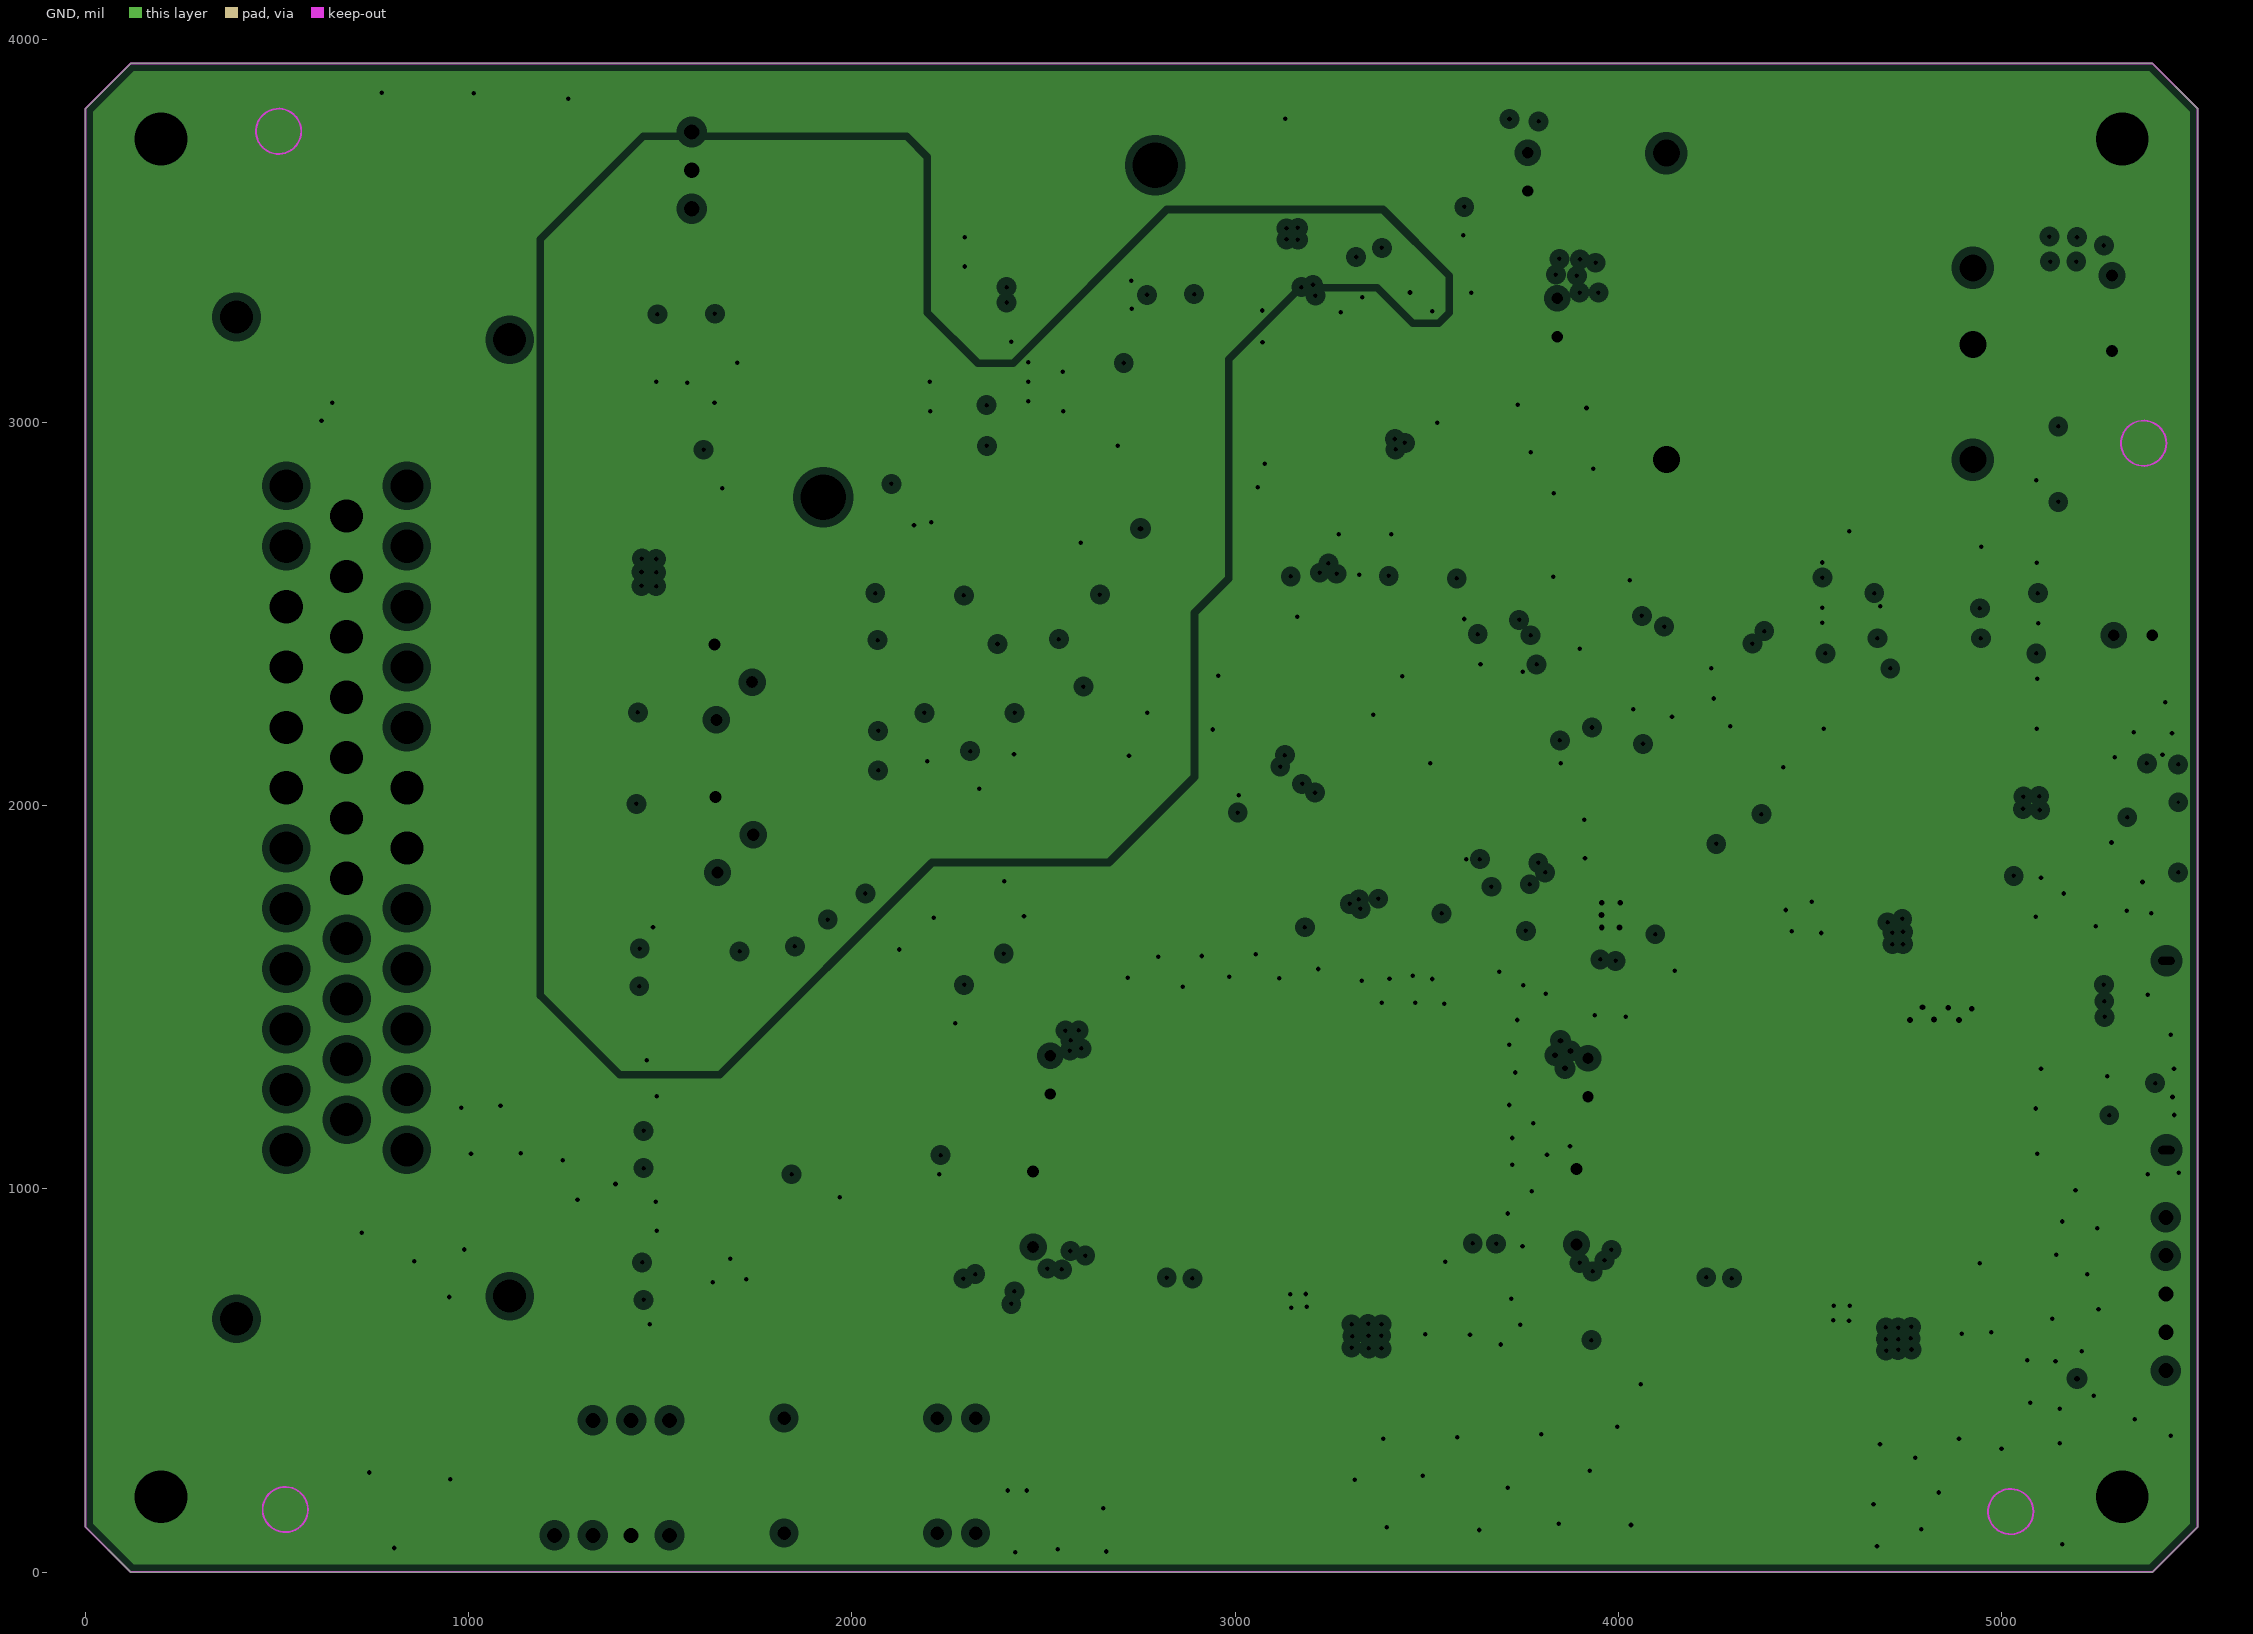
[diagram p0: GND, clearances drawn from the general rule]
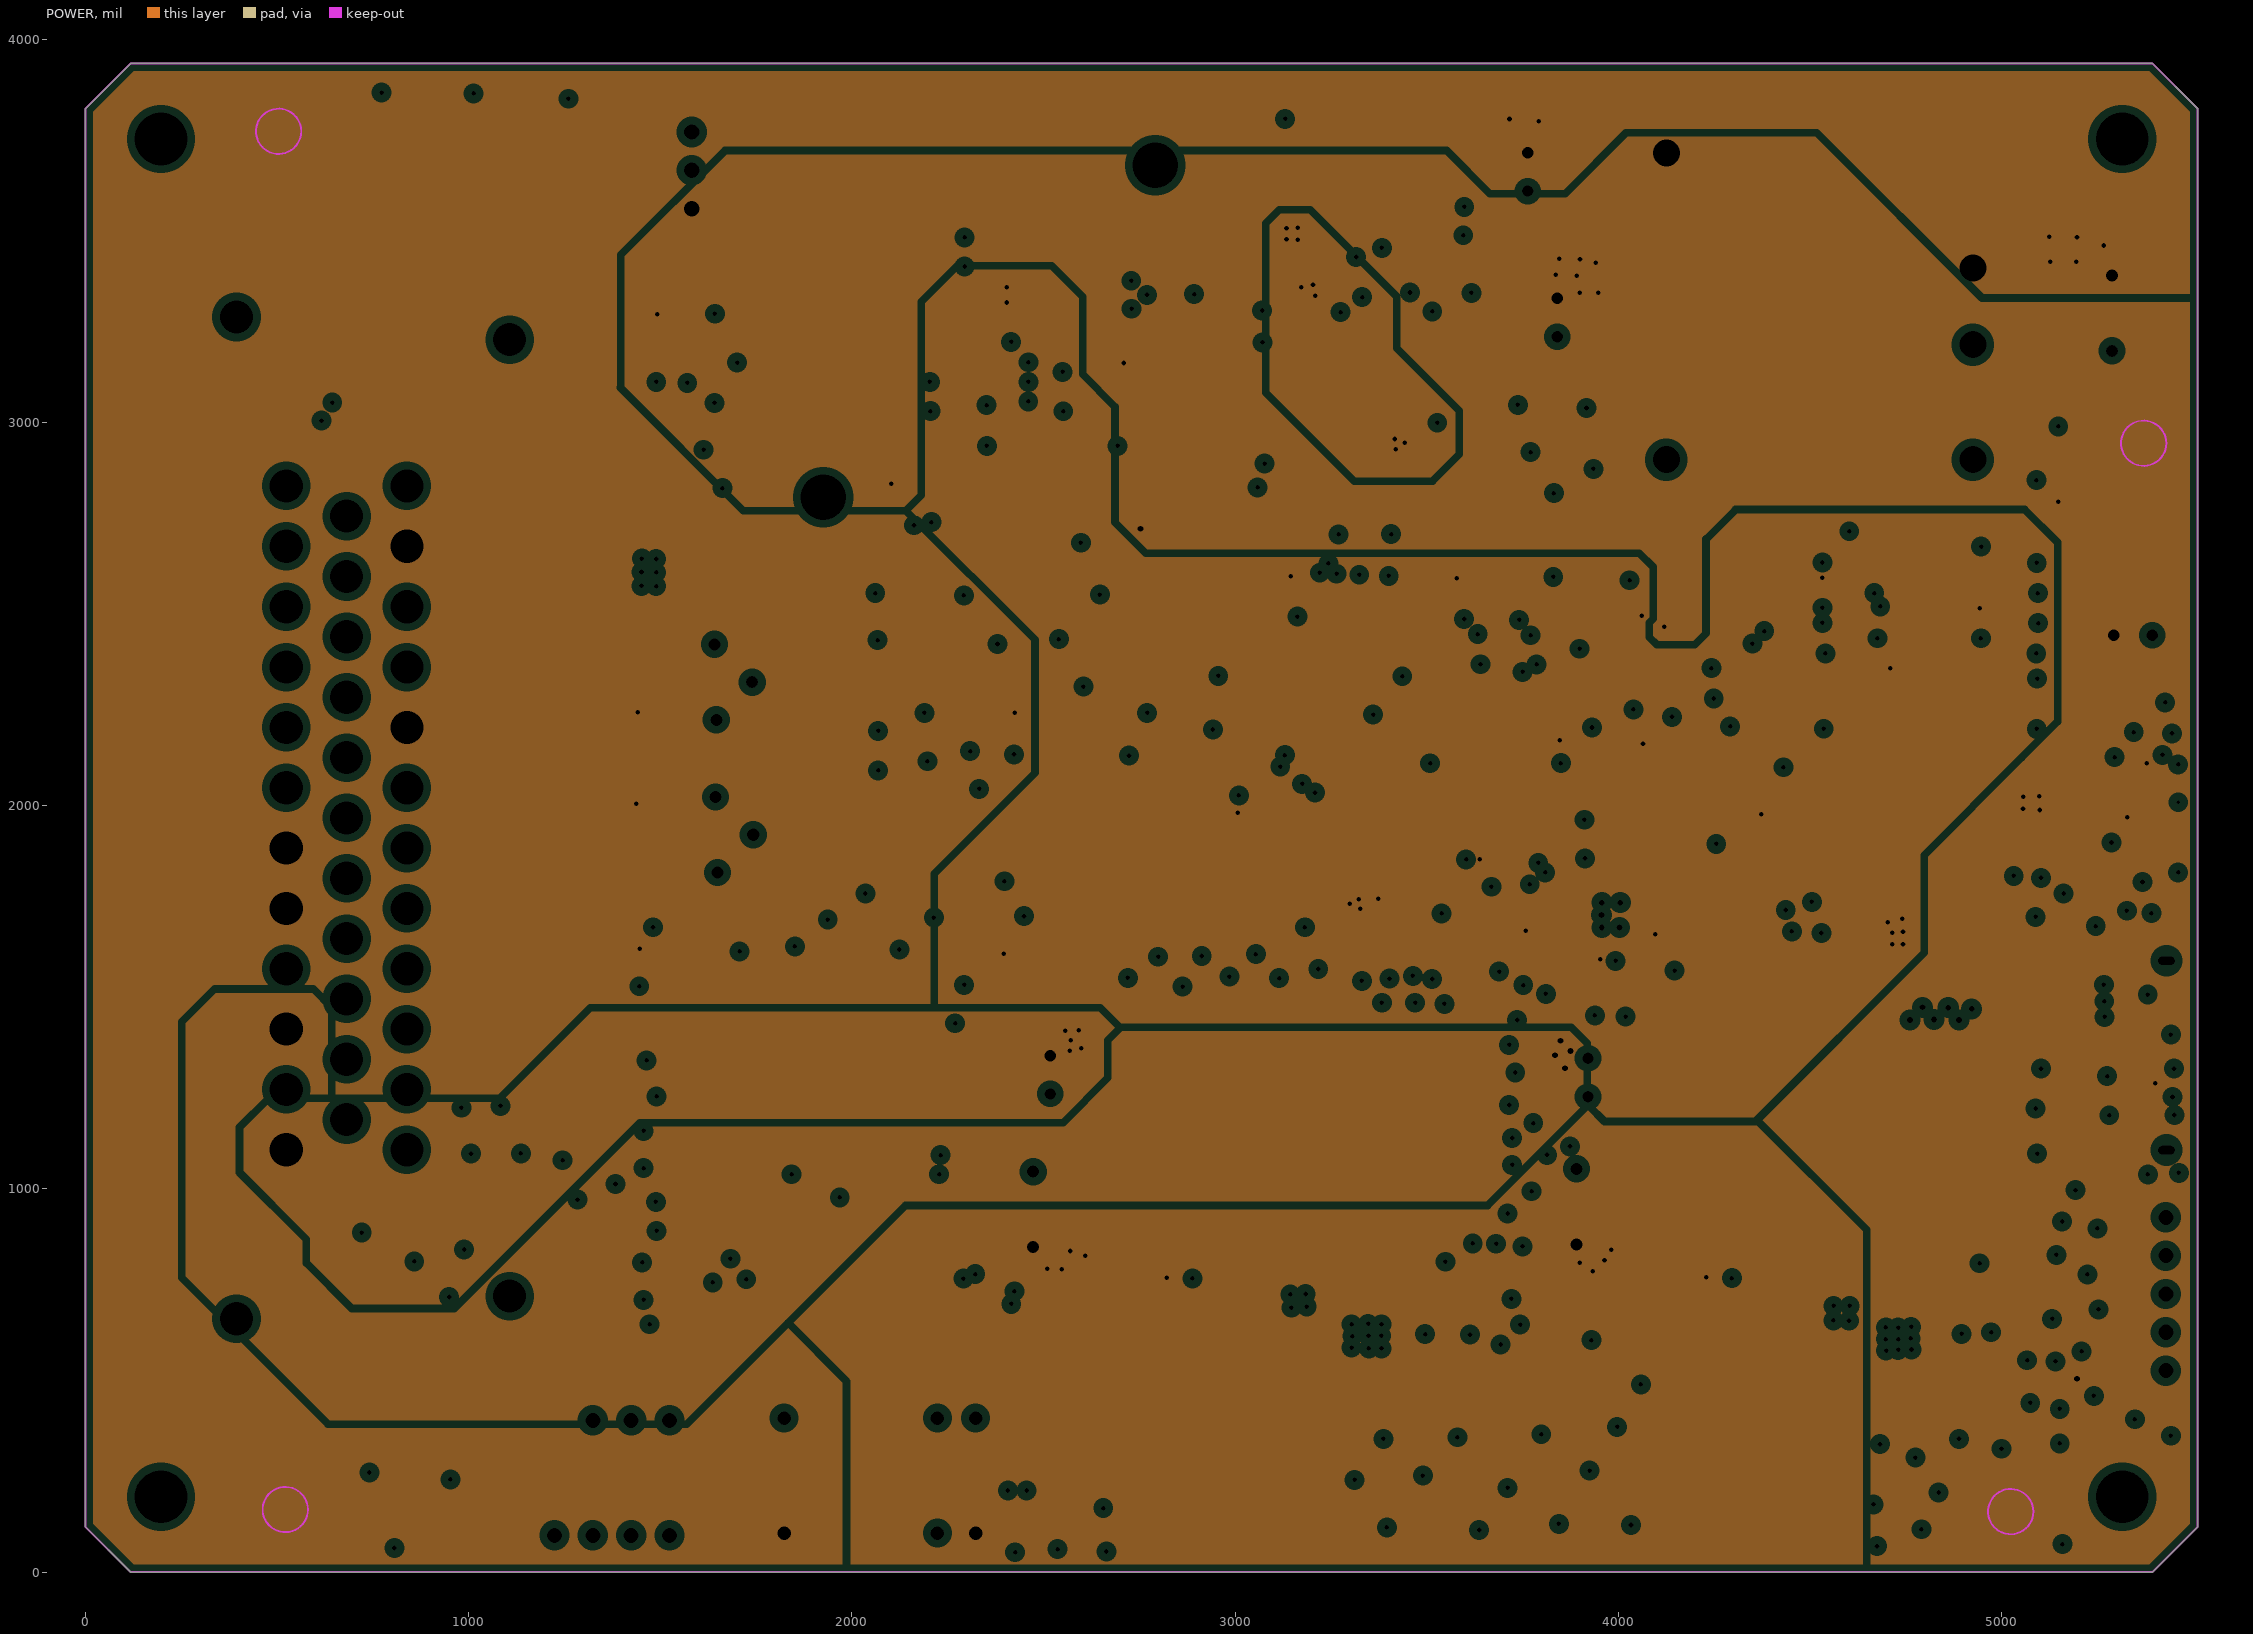
[diagram p1: POWER, clearances drawn from the general rule]
# Altium PCB MISC82155.PcbDoc (part 2 of 5)
## Footprints (in the part's own frame and the unit in brackets; to place one, negate y for a bottom-side part, rotate by r counter-clockwise, add the part's x,y. Pads: shape width x height; smd on the part's side, far side on the other; paste and mask are expansions set on the pad) (continued)
CTM1051AM [mm]
  round 1.6 hole 1: 1(-3.81,-3.81) 2(-1.27,-3.81) 3(1.27,-3.81) 4(3.81,-3.81) 5(3.81,3.81) 6(1.27,3.81) 7(-1.27,3.81)
  silkscreen extent -6.35,-6.1 6.35,4.81
DO-214 [mm]
  rect 1.8x2.4 smd: 1(-2.3,0) 2(2.3,0)
  silkscreen extent -3.5,-1.9 3.8,1.9
E2403UHBDD [mm]
  round 2.5 hole 1.8: 1(-10.16,-2.54) 2(-10.16,2.54) 3(10.16,-10.16) 5(10.16,10.16) 6(-10.16,10.16)
  silkscreen extent -12.7,-12.7 12.7,12.7
HDR1X3 [mil]
  rect 60x70 hole 40: 1(-100,0)
  oval 60x70 hole 40: 2(0,0) 3(100,0)
  silkscreen extent -175,-84 150,50, body extent -150,-50 150,50, height 298
HDR1X5 [mm]
  rect 1.6x1.6 hole 1: 1(-5.08,0)
  round 1.6 hole 1: 2(-2.54,0) 3(0,0) 4(2.54,0) 5(5.08,0)
  silkscreen extent -6.18,-1.1 6.18,1.1
HK4100F [mm]
  round 1.6 hole 0.9: 1(12.7,7.62) 2(0,7.62) 3(0,0) 4(2.54,7.62) 5(2.54,0) 6(12.7,0)
  silkscreen extent -1.27,-1.27 13.97,8.89
HOLE-3.2 [mm]
  round 5.6 hole 3.5: 8(0,0)
IC-24P-TSSOP-6_4MM-G [mil]
  rect 12x50 smd: 1(-140.75,-125) 2(-115.16,-125) 3(-89.57,-125) 4(-63.98,-125) 5(-38.39,-125) 6(-12.8,-125) 7(12.8,-125) 8(38.39,-125) 9(63.98,-125) 10(89.57,-125) 11(115.16,-125) 12(140.75,-125) 13(140.75,125) 14(115.16,125) 15(89.57,125) 16(63.98,125) 17(38.39,125) 18(12.8,125) 19(-12.8,125) 20(-38.39,125) 21(-63.98,125) 22(-89.57,125) 23(-115.16,125) 24(-140.75,125)
  silkscreen extent -177,-86 177,86
LC-SOT-23(SOT-23-3) [mm]
  rect 1.25x0.7 smd: 1(1.25,-0.95) 2(1.25,0.95) 3(-1.25,0)
  silkscreen extent -0.65,-1.46 0.9,1.46, body extent -1.5,-1.5 1.5,1.5, height 1.3
LED0805 [mm]
  rect 1.2x1.5 smd: 1(-1.1,0) 2(1.1,0)
  silkscreen extent -2.9,-1.1 1.95,1.4, body extent -1.02,-0.64 1.02,0.64, height 0.56
"Micro USB3.0-B" [mm]
  rect 1.1x1.7 hole 0.55 slot 1.1 at 90 deg: 0(0,0) 0(12.55,0)
  rect 0.4x1.35 smd: 1(2.31,2.7) 2(2.96,2.7) 3(3.61,2.7) 4(4.26,2.703) 5(4.91,2.718) 6(9.01,2.7) 7(9.66,2.7) 8(10.31,2.7) 9(10.96,2.7) 10(11.61,2.7)
  silkscreen extent -0.49,-2.65 12.76,2.93, body extent -0.36,-2.78 12.93,3.12, height 2.69
QFN24 [mm] "QFN, 24-Leads, Body 4.0x4.0mm (max), Pitch 0.50mm, IPC Medium Density"
  oval 0.65x0.25 smd: 1(-2.025,1.25) 2(-2.025,0.75) 3(-2.025,0.25) 4(-2.025,-0.25) 5(-2.025,-0.75) 6(-2.025,-1.25) 13(2.025,-1.25) 14(2.025,-0.75) 15(2.025,-0.25) 16(2.025,0.25) 17(2.025,0.75) 18(2.025,1.25)
  rect 2.5x2.5 smd: 1(0,0)
  oval 0.25x0.65 smd: 7(-1.25,-2.025) 8(-0.75,-2.025) 9(-0.25,-2.025) 10(0.25,-2.025) 11(0.75,-2.025) 12(1.25,-2.025) 19(1.25,2.025) 20(0.75,2.025) 21(0.25,2.025) 22(-0.25,2.025) 23(-0.75,2.025) 24(-1.25,2.025)
  silkscreen extent -3.02,-2 2,2, body extent -2,-2 2,2, height 0.9
QFP-100 [mm]
  rect 1.6x0.254 smd: 1(-8,6)
  oval 1.6x0.254 smd: 2(-8,5.5) 3(-8,5) 4(-8,4.5) 5(-8,4) 6(-8,3.5) 7(-8,3) 8(-8,2.5) 9(-8,2) 10(-8,1.5) 11(-8,1) 12(-8,0.5) 13(-8,0) 14(-8,-0.5) 15(-8,-1) 16(-8,-1.5) 17(-8,-2) 18(-8,-2.5) 19(-8,-3) 20(-8,-3.5) 21(-8,-4) 22(-8,-4.5) 23(-8,-5) 24(-8,-5.5) 25(-8,-6) 51(8,-6) 52(8,-5.5) 53(8,-5) 54(8,-4.5) 55(8,-4) 56(8,-3.5) 57(8,-3) 58(8,-2.5) 59(8,-2) 60(8,-1.5) 61(8,-1) 62(8,-0.5) 63(8,0) 64(8,0.5) 65(8,1) 66(8,1.5) 67(8,2) 68(8,2.5) 69(8,3) 70(8,3.5) 71(8,4) 72(8,4.5) 73(8,5) 74(8,5.5) 75(8,6)
  oval 0.254x1.6 smd: 26(-6,-8) 27(-5.5,-8) 28(-5,-8) 29(-4.5,-8) 30(-4,-8) 31(-3.5,-8) 32(-3,-8) 33(-2.5,-8) 34(-2,-8) 35(-1.5,-8) 36(-1,-8) 37(-0.5,-8) 38(0,-8) 39(0.5,-8) 40(1,-8) 41(1.5,-8) 42(2,-8) 43(2.5,-8) 44(3,-8) 45(3.5,-8) 46(4,-8) 47(4.5,-8) 48(5,-8) 49(5.5,-8) 50(6,-8) 76(6,8) 77(5.5,8) 78(5,8) 79(4.5,8) 80(4,8) 81(3.5,8) 82(3,8) 83(2.5,8) 84(2,8) 85(1.5,8) 86(1,8) 87(0.5,8) 88(0,8) 89(-0.5,8) 90(-1,8) 91(-1.5,8) 92(-2,8) 93(-2.5,8) 94(-3,8) 95(-3.5,8) 96(-4,8) 97(-4.5,8) 98(-5,8) 99(-5.5,8) 100(-6,8)
  silkscreen extent -9.07,-9.07 9.07,9.07
R0805 [mm]
  rect 1.2x1.4 smd: 1(-1,0) 2(1,0)
  silkscreen extent -2.05,-1.05 2.05,1.05, body extent -1.02,-0.65 1.02,0.62, height 0.61
R1210 [mm]
  rect 1.6x2.7 smd: 1(-1.4,0) 2(1.4,0)
  silkscreen extent -2.6,-1.75 2.6,1.75
R2512 [mm]
  rect 1.8x3.2 smd: 1(-2.8,0) 2(2.8,0)
  silkscreen extent -4.1,-2 4.1,2, body extent -3.18,-1.53 3.18,1.53, height 0.61
RB6.3*7 [mm]
  round 1.35 hole 0.75: 1(-1.27,0) 2(1.27,0)
  silkscreen extent -3.3,-3.3 3.33,3.3
SCC2130D [mm] "SOP, 24-Leads, Body 15.00x8.50mm, Pitch 1.00mm, IPC Medium Density"
  oval 2.25x0.7 smd: 1(-5.375,5.5) 2(-5.375,4.5) 3(-5.375,3.5) 4(-5.375,2.5) 5(-5.375,1.5) 6(-5.375,0.5) 7(-5.375,-0.5) 8(-5.375,-1.5) 9(-5.375,-2.5) 10(-5.375,-3.5) 11(-5.375,-4.5) 12(-5.375,-5.5) 13(5.375,-5.5) 14(5.375,-4.5) 15(5.375,-3.5) 16(5.375,-2.5) 17(5.375,-1.5) 18(5.375,-0.5) 19(5.375,0.5) 20(5.375,1.5) 21(5.375,2.5) 22(5.375,3.5) 23(5.375,4.5) 24(5.375,5.5)
  silkscreen extent -5.5,-7.5 3.85,7.5, body extent -4.25,-7.5 4.25,7.5, height 4.2
SLF12555 [mm] "TDK SMD power inductor"
  rect 3x3 smd: 1(-5.75,0) 2(5.75,0)
  silkscreen extent -6.25,-6.25 6.25,6.25
SMC [mm] "DO-214-AB/SMC; 2 C-Bend Leads; Body 7.9 x 5.9 mm, inc. leads (LxW)"
  rect 2.4x3.3 smd: 1(-3.475,0) 2(3.475,0)
  silkscreen extent -5.07,-2.05 5.43,2.05
SMD-4 [mm]
  rect 2x1.5 smd: 1(-4.65,1.27) 2(-4.65,-1.27) 3(4.65,-1.27) 4(4.65,1.27)
  silkscreen extent -5.4,-2.2 3,3, body extent -5.02,-2.42 5.01,2.42, height 3.9
SMD-D4148 [mil]
  rect 50x59.05 smd: 1(-60,0) 2(60,0)
  silkscreen extent -95,-35 106,35
SOP16-6.6 [mil]
  rect 80x24 smd: 1(-130,175) 2(-130,125) 3(-130,75) 4(-130,25) 5(-130,-25) 6(-130,-75) 7(-130,-125) 8(-130,-175) 9(130,-175) 10(130,-125) 11(130,-75) 12(130,-25) 13(130,25) 14(130,75) 15(130,125) 16(130,175)
  silkscreen extent -76,-205 76,205
SOP-8 [mil]
  rect 24x74 smd: 1(-75,-113)
  oval 24x74 smd: 2(-25,-113) 3(25,-113) 4(75,-113) 5(75,113) 6(25,113) 7(-25,113) 8(-75,113)
  silkscreen extent -95,-65 95,65
SOT-23 [mil]
  rect 40x36 smd: 1(-42.5,37.4) 2(-42.5,-37.4) 3(42.5,0)
  silkscreen extent -25,-56 25,56, body extent -47,-57 50,58, height 39
SOT-223 [mm]
  rect 1.1x2.15 smd: 1(-2.3,-3.1) 2(0,-3.1) 3(2.3,-3.1)
  rect 3.5x2.15 smd: 2(0,3.1)
  silkscreen extent -3.35,-4.85 3.35,1.63, body extent -3.15,-3.3 3.15,3.3, height 1.8
TO-252 [mm] "DPAK"
  rect 1.524x2.28 smd: 1(-2.2,0) 1(2.2,0)
  rect 6.74x6.23 smd: 2(0,8.14)
  silkscreen extent -4,2.05 4.05,11.95, body extent -3.24,-0.5 3.26,10.5, height 2.2
TO-263-5 [mm]
  rect 8.4x10.65 smd: 0(-10.3,0)
  rect 3.8x1.05 smd: 1(0,-3.4) 2(0,-1.7) 3(0,0) 4(0,1.7) 5(0,3.4)
  silkscreen extent -5.65,-5.35 -2.1,5.35
VGA35 [mm]
  round 3 hole 2.2: 1(-22,2.25) 2(-18,2.25) 3(-14,2.25) 4(-10,2.25) 5(-6,2.25) 6(-2,2.25) 7(2,2.25) 8(6,2.25) 9(10,2.25) 10(14,2.25) 11(18,2.25) 12(22,2.25) 13(-20,-1.75) 14(-16,-1.75) 15(-12,-1.75) 16(-8,-1.75) 17(-4,-1.75) 18(0,-1.75) 19(4,-1.75) 20(8,-1.75) 21(12,-1.75) 22(16,-1.75) 23(20,-1.75) 24(-22,-5.75) 25(-18,-5.75) 26(-14,-5.75) 27(-10,-5.75) 28(-6,-5.75) 29(-2,-5.75) 30(2,-5.75) 31(6,-5.75) 32(10,-5.75) 33(14,-5.75) 34(18,-5.75) 35(22,-5.75) 36(-31.7,9.05) 37(31.7,9.05) 38(33.2,-9.05) 39(-33.2,-9.05)
  silkscreen extent -38.45,-17.87 38.48,14.36
XTAL7050 [mm]
  rect 2x1.8 smd: 1(-2.54,-2.1) 2(2.54,-2.1) 3(2.54,2.1) 4(-2.54,2.1)
  silkscreen extent -4.37,-3.85 4,3.5

## Part data
C1 C6 C8 C10 C31 C35 C61 C62 C68: library part "Cap Pol2", "Polarized Capacitor (Axial)"
C2 C3 C4 C5 C7 C9 C11 C12 C13 C14 C15 C16 C17 C22 C28 C36 C37 C39 C41 C42 C44 C45 C46 C47 C48 C49 C50 C51 C52 C53 C54 C55 C56 C57 C58 C59 C60 C63 C64 C65 C66 C67 C70 C71 C72 C73 C74 C75 C76 C77 C78: library part Cap, "Capacitor"
C18 C33 C40: library part 1.02.11.0018, "220μF,16V,Φ6.3×7mm,,Zhuhai Huaguan,RoHS"
C19 C20 C21 C32 C34 C38 C43 C69: library part "CAP NP_Dup5"
C23 C24 C25 C26 C27 C29 C30: library part CAP, "Capacitor"
D1 D2 D3 D5: library part LED0, "Typical INFRARED GaAs LED"
D4 D10 D11: library part "D Zener", "Zener Diode"
D6 D7 D8 D9 D12: library part "Diode 1N4007", "1 Amp General Purpose Rectifier"
D13: library part Diode, "Default Diode"
DW3 DW4: library part ZENER3, "Zener Diode"
K1: library part Relay-SPDT, "Single-Pole Dual-Throw Relay"
L1 L2 L3 L4 L5 L6: library part Inductor, "Inductor"
P1: library part "Header 18X2", "Header, 18-Pin, Dual row"
P4: library part "Header 5", "Header, 5-Pin"
Q1: library part 1.04.09.0001, "SS8050LT(1.5A),SOT-23,Jiangsu Changdian,RoHS"
Q2: library part PNP, "PNP Bipolar Transistor"
R1 R2 R4 R5 R7 R10 R13 R14 R15 R16 R17 R18 R19 R20 R21 R22 R24 R25 R26 R27 R28 R29 R30 R31 R32 R34 R35 R36 R37 R38 R39 R40 R41 R42 R43 R44 R45 R46 R47 R48 R49 R54 R55 R56 R57 R58 R59 R60 R61 R62 U2/: library part Res, "Resistor"
R3 R50: library part RES
R6 R8 R9 R11 R12: library part 1.01.17.0004
R23 R33: library part "Res Adj1", "Variable Resistor"
U1: library part AD7190
U2: library part "Header 3", "Header, 3-Pin"
U3: library part ITG3050, "3-axi gyros"
U4: library part E2403UHBDD-10W
U5 U19: library part VOLTREG1
U6: library part ADR03ARZ
U7: library part TLP281-1, "Optoisolator"
U8: library part STM32F103VBH6
U10: library part LM293D, "Dual Comparator"
U13 U14: library part LM358D, "Dual Low-Power Operational Amplifier"
U15: library part TL431A, "TL431A"
U16: library part SP202ECT
U17 U18: library part PESD12VL2BT
Y1: library part "Header 2X2", "Header, 2-Pin, Dual row"

## Free pads (board coordinates)
  round 39.37 smd mask+39.37: 0(504,3760) 0(521.41,163.34) 0(5024,158) 0(5371,2946)
  round 39.37 smd far side mask+39.37: 0(504,3760) 0(521.41,163.34) 0(5024,158) 0(5371,2946)

## Via types
v1: diameter 24, hole 12, Top Layer to Bottom Layer, 278 vias
v2: diameter 23.62, hole 11.81, Top Layer to Bottom Layer, 144 vias
v3: diameter 30, hole 15, Top Layer to Bottom Layer, 17 vias
v4: diameter 20, hole 10, Top Layer to Bottom Layer, 1 vias

## Nets (pads, with @x,y where several pads share a name; then routed paths per layer and width w, separated by ;. In a path a pad name is that pad's centre, name@x,y a point inside that pad or via, vN(x,y) a via of type N, cw(c..) or ccw(c..) an arc to the next point about the centre after c; other vN are vias at no path point)
646_OUT: C60.1 R49.2 U20.A2 U20.B1 | length 2441.6
  Top Layer w20: R49.2@2051,3517.37 2150.37,3517.37 2238,3605 2480,3605 2521,3564 2814,3564 2962,3416 2962,3114 3215,2861 3510,2861 3616.41,2967.41 C60.1@3616.41,3084 ; U20.A2@3456.4,3106.85 U20.B1@3487.89,3138.35 3534.4,3138.35 3588.75,3084 C60.1@3615,3084
6050_INT: U3.12 U8.98 | length 784.7
  Top Layer w6: U8.98@3578.26,1916.38 3578.26,1849.69 3592.61,1835.34 3592.66,1835.34 3598,1830 3773,1830 3812,1791 3851,1791 3869,1773 3869,1610 3910,1569 4010,1569 4032.21,1591.21 U3.12@4032.21,1634.28